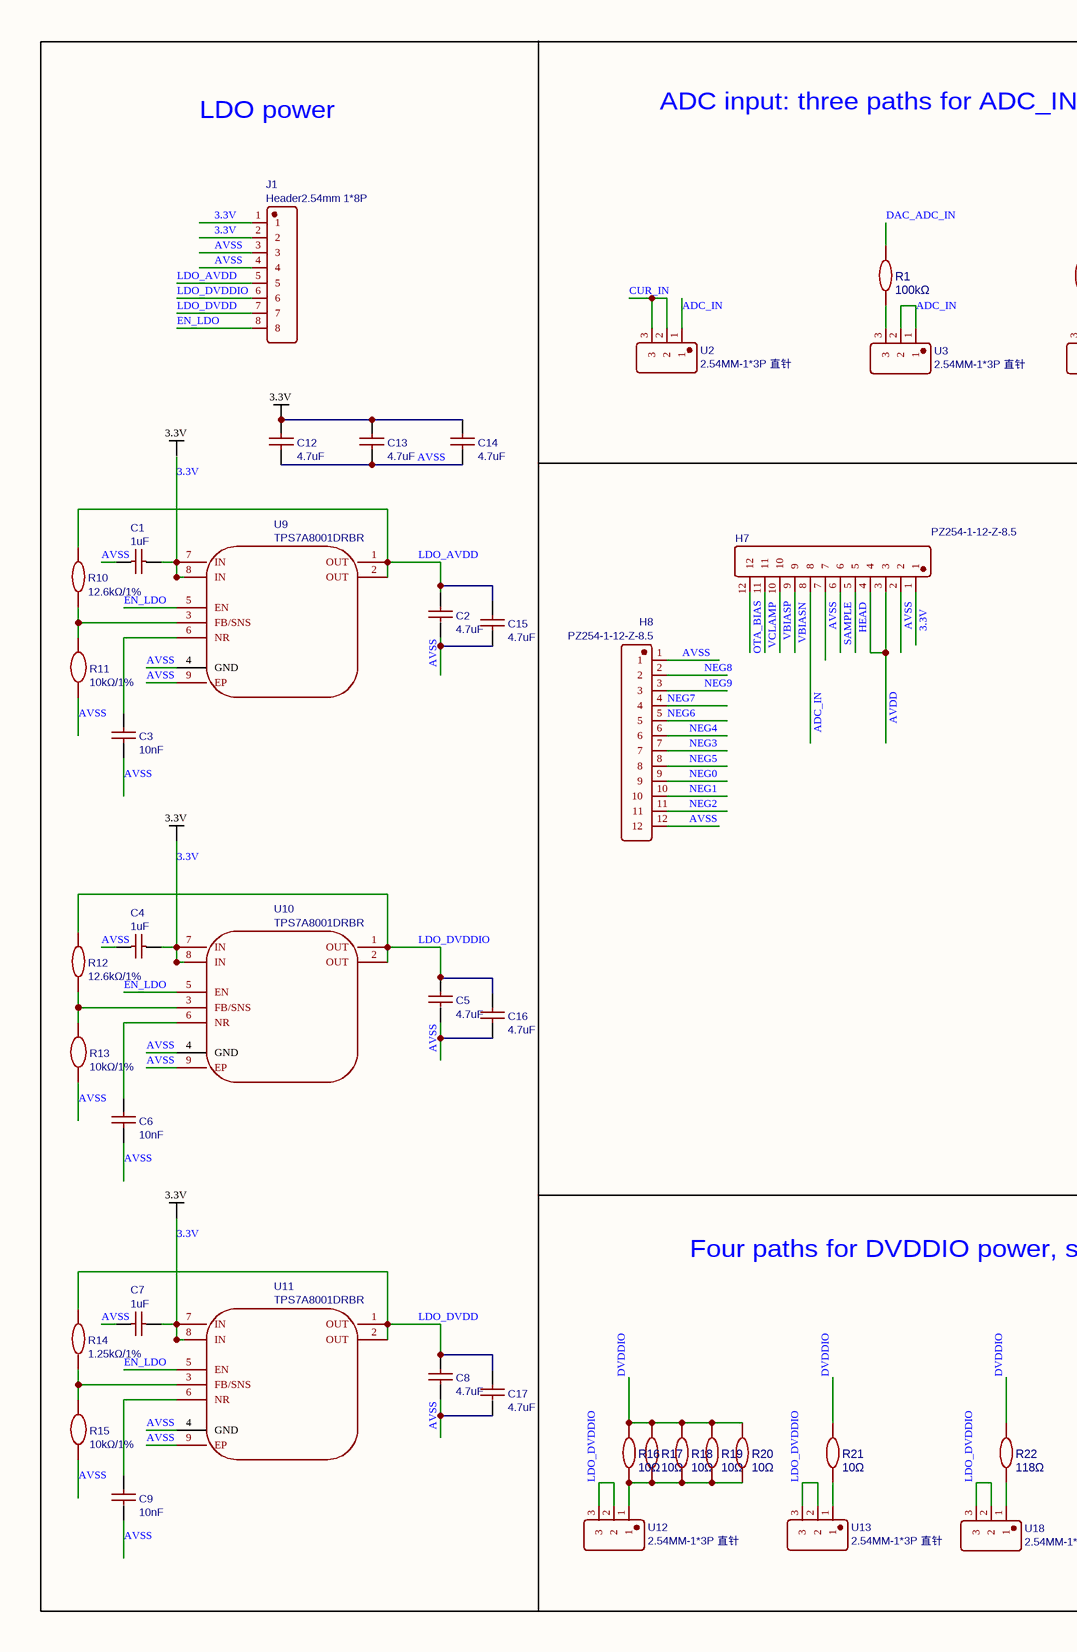
[diagram p0: MISC79022-11.schdoc, left]
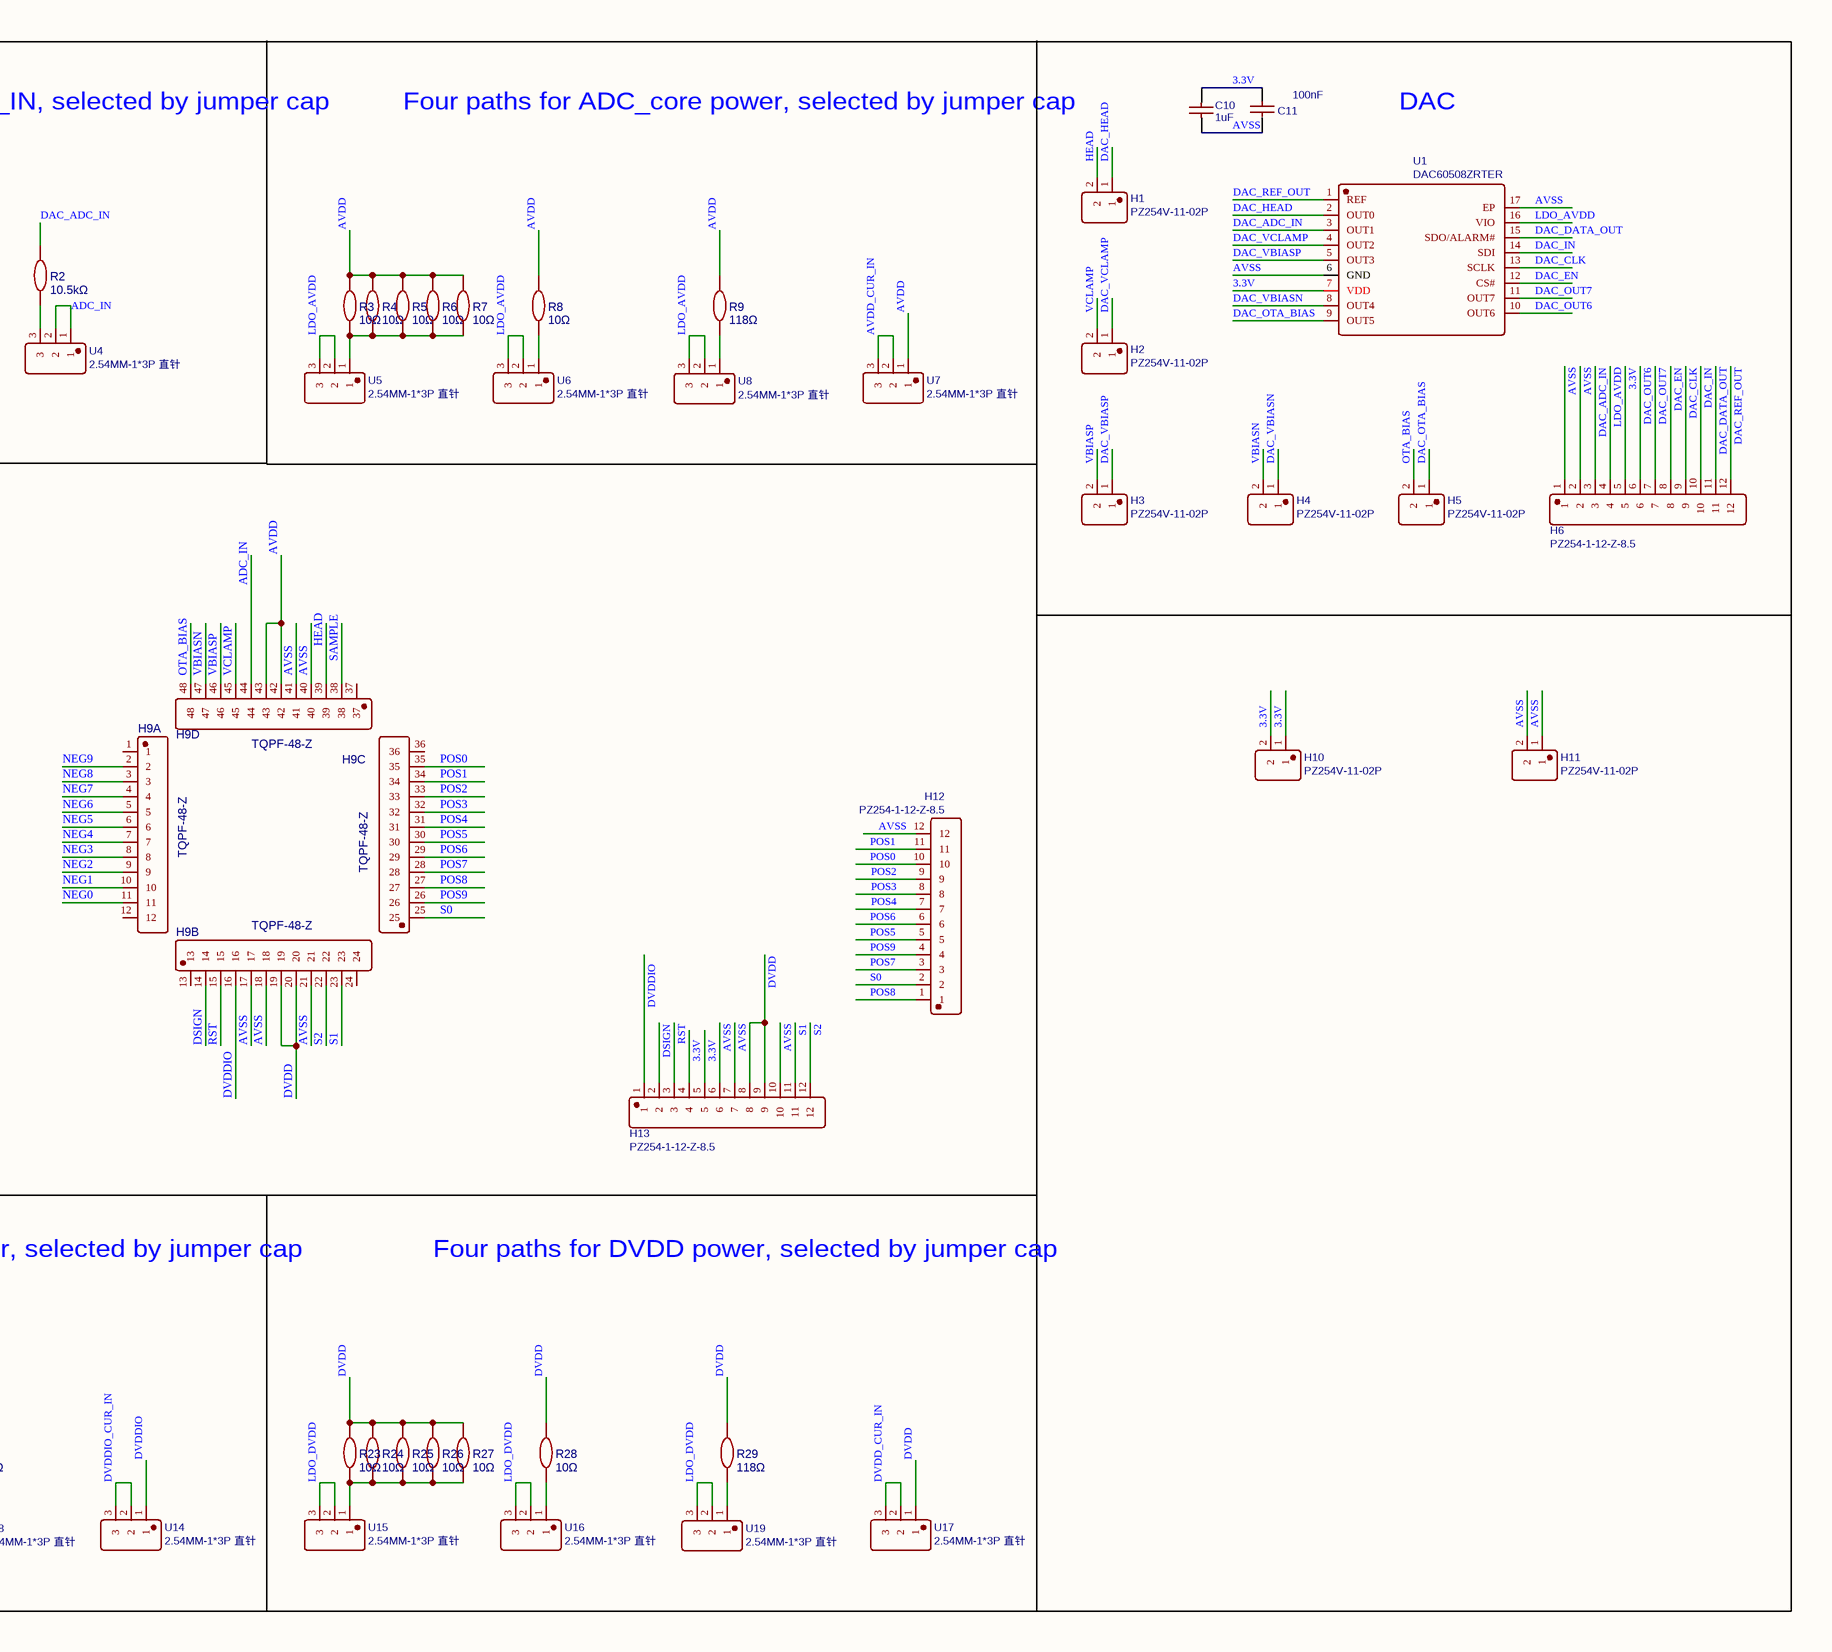
[diagram p1: MISC79022-11.schdoc, right]
# Altium project MISC79022-5.PrjPCB
1 sheet, 79 parts. Net scope: global (net labels, ports and power ports of the same name join across sheets).
Board file: MISC79022.pcbdoc

## Sheet MISC79022-11.schdoc
size 490 x 284 mm

### Parts
C1  1uF  [C0603]
C2  4.7uF  [C0603]
C3  10nF  [C0603]
C4  1uF  [C0603]
C5  4.7uF  [C0603]
C6  10nF  [C0603]
C7  1uF  [C0603]
C8  4.7uF  [C0603]
C9  10nF  [C0603]
C10  1uF  [C0603]
C11  100nF  [C0603]
C12  4.7uF  [C0603]
C13  4.7uF  [C0603]
C14  4.7uF  [C0603]
C15  4.7uF  [C0603]
C16  4.7uF  [C0603]
C17  4.7uF  [C0603]
H1  PZ254V-11-02P  [HDR-TH_2P-P2.54-V-M]
H2  PZ254V-11-02P  [HDR-TH_2P-P2.54-V-M]
H3  PZ254V-11-02P  [HDR-TH_2P-P2.54-V-M]
H4  PZ254V-11-02P  [HDR-TH_2P-P2.54-V-M]
H5  PZ254V-11-02P  [HDR-TH_2P-P2.54-V-M]
H6  PZ254-1-12-Z-8.5  [HDR-TH_12P-P2.54-V-M]
H7  PZ254-1-12-Z-8.5  [HDR-TH_12P-P2.54-V-M]
H8  PZ254-1-12-Z-8.5  [HDR-TH_12P-P2.54-V-M]
H9  TQPF-48-Z  [TQPF-48-Z]  (parts A,B,C,D of 4)
H10  PZ254V-11-02P  [HDR-TH_2P-P2.54-V-M]
H11  PZ254V-11-02P  [HDR-TH_2P-P2.54-V-M]
H12  PZ254-1-12-Z-8.5  [HDR-TH_12P-P2.54-V-M]
H13  PZ254-1-12-Z-8.5  [HDR-TH_12P-P2.54-V-M]
J1  Header2.54mm 1*8P  [HDR-TH_8P-P2.54-V-M]
R1  100kΩ  [R0805]
R2  10.5kΩ  [R0603]
R3  10Ω  [R1206]
R4  10Ω  [R1206]
R5  10Ω  [R1206]
R6  10Ω  [R1206]
R7  10Ω  [R1206]
R8  10Ω  [R1206]
R9  118Ω  [R0603]
R10  12.6kΩ/1%  [R0603]
R11  10kΩ/1%  [R0603]
R12  12.6kΩ/1%  [R0603]
R13  10kΩ/1%  [R0603]
R14  1.25kΩ/1%  [R0805]
R15  10kΩ/1%  [R0603]
R16  10Ω  [R1206]
R17  10Ω  [R1206]
R18  10Ω  [R1206]
R19  10Ω  [R1206]
R20  10Ω  [R1206]
R21  10Ω  [R1206]
R22  118Ω  [R0603]
R23  10Ω  [R1206]
R24  10Ω  [R1206]
R25  10Ω  [R1206]
R26  10Ω  [R1206]
R27  10Ω  [R1206]
R28  10Ω  [R1206]
R29  118Ω  [R0603]
U1  DAC60508ZRTER  [WQFN-16_L3.0-W3.0-P0.50-BL-EP0.8]
U2  2.54MM-1*3P 直针  [HDR-TH_3P-P2.54-V-M-1]
U3  2.54MM-1*3P 直针  [HDR-TH_3P-P2.54-V-M-1]
U4  2.54MM-1*3P 直针  [HDR-TH_3P-P2.54-V-M-1]
U5  2.54MM-1*3P 直针  [HDR-TH_3P-P2.54-V-M-1]
U6  2.54MM-1*3P 直针  [HDR-TH_3P-P2.54-V-M-1]
U7  2.54MM-1*3P 直针  [HDR-TH_3P-P2.54-V-M-1]
U8  2.54MM-1*3P 直针  [HDR-TH_3P-P2.54-V-M-1]
U9  TPS7A8001DRBR  [VSON-8_L3.0-W3.0-P0.65-TL-EP]
U10  TPS7A8001DRBR  [VSON-8_L3.0-W3.0-P0.65-TL-EP]
U11  TPS7A8001DRBR  [VSON-8_L3.0-W3.0-P0.65-TL-EP]
U12  2.54MM-1*3P 直针  [HDR-TH_3P-P2.54-V-M-1]
U13  2.54MM-1*3P 直针  [HDR-TH_3P-P2.54-V-M-1]
U14  2.54MM-1*3P 直针  [HDR-TH_3P-P2.54-V-M-1]
U15  2.54MM-1*3P 直针  [HDR-TH_3P-P2.54-V-M-1]
U16  2.54MM-1*3P 直针  [HDR-TH_3P-P2.54-V-M-1]
U17  2.54MM-1*3P 直针  [HDR-TH_3P-P2.54-V-M-1]
U18  2.54MM-1*3P 直针  [HDR-TH_3P-P2.54-V-M-1]
U19  2.54MM-1*3P 直针  [HDR-TH_3P-P2.54-V-M-1]

### Nets
3.3V: C1.1 C4.1 C7.1 C10.1 C11.2 C12.2 C13.2 C14.2 H6.5 H7.1 H10.1 H10.2 H13.4 H13.5 J1.1 J1.2 U1.7(VDD) U9.7(IN) U9.8(IN) U10.7(IN) U10.8(IN) U11.7(IN) U11.8(IN)
ADC_IN: H7.8 H9.44 U2.1 U3.1 U3.2 U4.1 U4.2
AVDD: H7.3 H7.4 H9.42 H9.43 R3.2 R4.2 R5.2 R6.2 R7.2 R8.2 R9.2 U7.1
AVDD_CUR_IN: U7.2 U7.3
AVSS: C1.2 C2.1 C3.1 C4.2 C5.1 C6.1 C7.2 C8.1 C9.1 C10.2 C11.1 C12.1 C13.1 C14.1 C15.1 C16.1 C17.1 H6.1 H6.2 H7.2 H7.7 H8.1 H8.12 H9.17 H9.18 H9.21 H9.40 H9.41 H11.1 H11.2 H12.12 H13.6 H13.7 H13.10 J1.3 J1.4 R11.1 R13.1 R15.1 U1.6(GND) U1.17(EP) U9.4(GND) U9.9(EP) U10.4(GND) U10.9(EP) U11.4(GND) U11.9(EP)
CUR_IN: U2.2 U2.3
DAC_ADC_IN: H6.3 R1.2 R2.2 U1.3(OUT1)
DAC_CLK: H6.9 U1.13(SCLK)
DAC_DATA_OUT: H6.11 U1.15(SDO/ALARM#)
DAC_EN: H6.8 U1.12(CS#)
DAC_HEAD: H1.1 U1.2(OUT0)
DAC_IN: H6.10 U1.14(SDI)
DAC_OTA_BIAS: H5.1 U1.9(OUT5)
DAC_OUT6: H6.6 U1.10(OUT6)
DAC_OUT7: H6.7 U1.11(OUT7)
DAC_REF_OUT: H6.12 U1.1(REF)
DAC_VBIASN: H4.1 U1.8(OUT4)
DAC_VBIASP: H3.1 U1.5(OUT3)
DAC_VCLAMP: H2.1 U1.4(OUT2)
DSIGN: H9.14 H13.2
DVDD: H9.19 H9.20 H13.8 H13.9 R23.2 R24.2 R25.2 R26.2 R27.2 R28.2 R29.2 U17.1
DVDD_CUR_IN: U17.2 U17.3
DVDDIO: H9.16 H13.1 R16.2 R17.2 R18.2 R19.2 R20.2 R21.2 R22.2 U14.1
DVDDIO_CUR_IN: U14.2 U14.3
EN_LDO: J1.8 U9.5(EN) U10.5(EN) U11.5(EN)
HEAD: H1.2 H7.5 H9.39
LDO_AVDD: C2.2 C15.2 H6.4 J1.5 R10.1 U1.16(VIO) U5.2 U5.3 U6.2 U6.3 U8.2 U8.3 U9.1(OUT) U9.2(OUT)
LDO_DVDD: C8.2 C17.2 J1.7 R14.1 U11.1(OUT) U11.2(OUT) U15.2 U15.3 U16.2 U16.3 U19.2 U19.3
LDO_DVDDIO: C5.2 C16.2 J1.6 R12.1 U10.1(OUT) U10.2(OUT) U12.2 U12.3 U13.2 U13.3 U18.2 U18.3
NEG0: H8.9 H9.11
NEG1: H8.10 H9.10
NEG2: H8.11 H9.9
NEG3: H8.7 H9.8
NEG4: H8.6 H9.7
NEG5: H8.8 H9.6
NEG6: H8.5 H9.5
NEG7: H8.4 H9.4
NEG8: H8.2 H9.3
NEG9: H8.3 H9.2
OTA_BIAS: H5.2 H7.12 H9.48
POS0: H9.35 H12.10
POS1: H9.34 H12.11
POS2: H9.33 H12.9
POS3: H9.32 H12.8
POS4: H9.31 H12.7
POS5: H9.30 H12.5
POS6: H9.29 H12.6
POS7: H9.28 H12.3
POS8: H9.27 H12.1
POS9: H9.26 H12.4
RST: H9.15 H13.3
S0: H9.25 H12.2
S1: H9.23 H13.11
S2: H9.22 H13.12
SAMPLE: H7.6 H9.38
VBIASN: H4.2 H7.9 H9.47
VBIASP: H3.2 H7.10 H9.46
VCLAMP: H2.2 H7.11 H9.45
NetC3_2: C3.2 U9.6(NR)
NetC6_2: C6.2 U10.6(NR)
NetC9_2: C9.2 U11.6(NR)
NetR1_1: R1.1 U3.3
NetR2_1: R2.1 U4.3
NetR3_1: R3.1 R4.1 R5.1 R6.1 R7.1 U5.1
NetR8_1: R8.1 U6.1
NetR9_1: R9.1 U8.1
NetR10_2: R10.2 R11.2 U9.3(FB/SNS)
NetR12_2: R12.2 R13.2 U10.3(FB/SNS)
NetR14_2: R14.2 R15.2 U11.3(FB/SNS)
NetR16_1: R16.1 R17.1 R18.1 R19.1 R20.1 U12.1
NetR21_1: R21.1 U13.1
NetR22_1: R22.1 U18.1
NetR23_1: R23.1 R24.1 R25.1 R26.1 R27.1 U15.1
NetR28_1: R28.1 U16.1
NetR29_1: R29.1 U19.1

Not connected (* = marked no-connect by the designer): H9 1 12 13 24 36 37

### Notes on the sheet
- LDO power
- ADC input: three paths for ADC_IN, selected by jumper cap
- Four paths for ADC_core power, selected by jumper cap
- DAC
- Four paths for DVDDIO power, selected by jumper cap
- Four paths for DVDD power, selected by jumper cap
- Labels drawn without touching a wire or pin: 3.3V

### Library data of the parts
C1 C4 C7 C10 = 1uF: Manufacturer Part: CL10A105KB8NNNC; Manufacturer: SAMSUNG(三星); nameAlias: Value; Supplier: LCSC; Supplier Part: C15849; JLCPCB Part Class: Basic Part; spicePre: C; spiceSymbolName: CL10A105KB8NNNC
C2 C5 C8 C12-C17 = 4.7uF: Manufacturer Part: CL10A475KO8NNNC; Manufacturer: SAMSUNG(三星); nameAlias: Value; Supplier: LCSC; Supplier Part: C19666; JLCPCB Part Class: Basic Part; spicePre: C; spiceSymbolName: CL10A475KO8NNNC
C3 C6 C9 C11 = 10nF: Manufacturer: YAGEO(国巨); Manufacturer Part: CC0603KRX7R9BB103; nameAlias: Value; Supplier: LCSC; Supplier Part: C100042; JLCPCB Part Class: Extended Part; spicePre: C; spiceSymbolName: CC0603KRX7R9BB103
H1-H5 H10 H11 = PZ254V-11-02P: Manufacturer: XFCN(兴飞); Contributor: LCSC; Supplier: LCSC; Supplier Part: C492401; Manufacturer Part: PZ254V-11-02P; JLCPCB Part Class: Extended Part; spicePre: H; spiceSymbolName: PZ254V-11-02P
H6-H9 H12 H13 = PZ254-1-12-Z-8.5: Manufacturer: HCTL(华灿天禄); Contributor: LCSC; Supplier: LCSC; Supplier Part: C2894935; Manufacturer Part: PZ254-1-12-Z-8.5; JLCPCB Part Class: Extended Part; spicePre: H; spiceSymbolName: PZ254-1-12-Z-8.5
J1 = Header2.54mm 1*8P: Manufacturer: null; Manufacturer Part: 直排针2.54mm 1*8P; Supplier Part: C49256; Supplier: LCSC; JLCPCB Part Class: Extended Part; spicePre: J; spiceSymbolName: Header2.54mm 1*8P
R1 = 100kΩ: Manufacturer: KAMAYA(釜屋電機); Manufacturer Part: RMC1/10-104JTP; nameAlias: Value; Contributor: LCSC; Supplier: LCSC; Supplier Part: C340475; JLCPCB Part Class: Extended Part; spicePre: R; spiceSymbolName: RMC1/10-104JTP
R2 = 10.5kΩ: Manufacturer: KOA; Manufacturer Part: RK73H1JTTD1052F; nameAlias: Value; Contributor: LCSC; Supplier: LCSC; Supplier Part: C317147; JLCPCB Part Class: Extended Part; spicePre: R; spiceSymbolName: RK73H1JTTD1052F
R3-R8 R16-R21 R23-R28 = 10Ω: Manufacturer: KOA; Manufacturer Part: RK73H2BTTD10R0F; nameAlias: Value; Contributor: LCSC; Supplier: LCSC; Supplier Part: C346120; JLCPCB Part Class: Extended Part; spicePre: R; spiceSymbolName: RK73H2BTTD10R0F
R9 R22 R29 = 118Ω: Manufacturer: KOA; Manufacturer Part: RK73H1JTTD1180F; nameAlias: Value; Contributor: LCSC; Supplier: LCSC; Supplier Part: C317095; JLCPCB Part Class: Extended Part; spicePre: R; spiceSymbolName: RK73H1JTTD1180F
R10 R12 = 12.6kΩ/1%: Manufacturer: VO(翔胜); Manufacturer Part: MF1/8W ±1% 12K5 OTB5; nameAlias: Value; Contributor: LCSC; Supplier: LCSC; Supplier Part: C337058; JLCPCB Part Class: Extended Part; spicePre: R; spiceSymbolName: MF1/8W ±1% 12K5 OTB5
R11 R13 R15 = 10kΩ/1%: Manufacturer: Viking(光颉); Manufacturer Part: ARG05BTC1002; nameAlias: Value; Contributor: LCSC; Supplier: LCSC; Supplier Part: C406725; JLCPCB Part Class: Extended Part; spicePre: R; spiceSymbolName: ARG05BTC1002
R14 = 1.25kΩ/1%: Manufacturer: VO(翔胜); Manufacturer Part: MF1/8W ±1% 12K5 OTB5; nameAlias: Value; Contributor: LCSC; Supplier: LCSC; Supplier Part: C337058; JLCPCB Part Class: Extended Part; spicePre: R; spiceSymbolName: MF1/8W ±1% 12K5 OTB5
U1 = DAC60508ZRTER: Manufacturer: TI(德州仪器); Contributor: LCSC; Supplier: LCSC; Supplier Part: C2679476; Manufacturer Part: DAC60508ZRTER; JLCPCB Part Class: Extended Part; spicePre: U; spiceSymbolName: DAC60508ZRTER
U2-U8 U12-U19 = 2.54MM-1*3P 直针: Manufacturer: null; Contributor: lcsc; Supplier: LCSC; Supplier Part: C9900025313; Manufacturer Part: 2.54mm-1*3P 直针; JLCPCB Part Class: Extended Part; spicePre: U; spiceSymbolName: 2.54MM-1*3P 直针
U9-U11 = TPS7A8001DRBR: Manufacturer: TI(德州仪器); Supplier: LCSC; Manufacturer Part: TPS7A8001DRBR; Supplier Part: C105265; JLCPCB Part Class: Extended Part; spicePre: U; spiceSymbolName: TPS7A8001DRBR